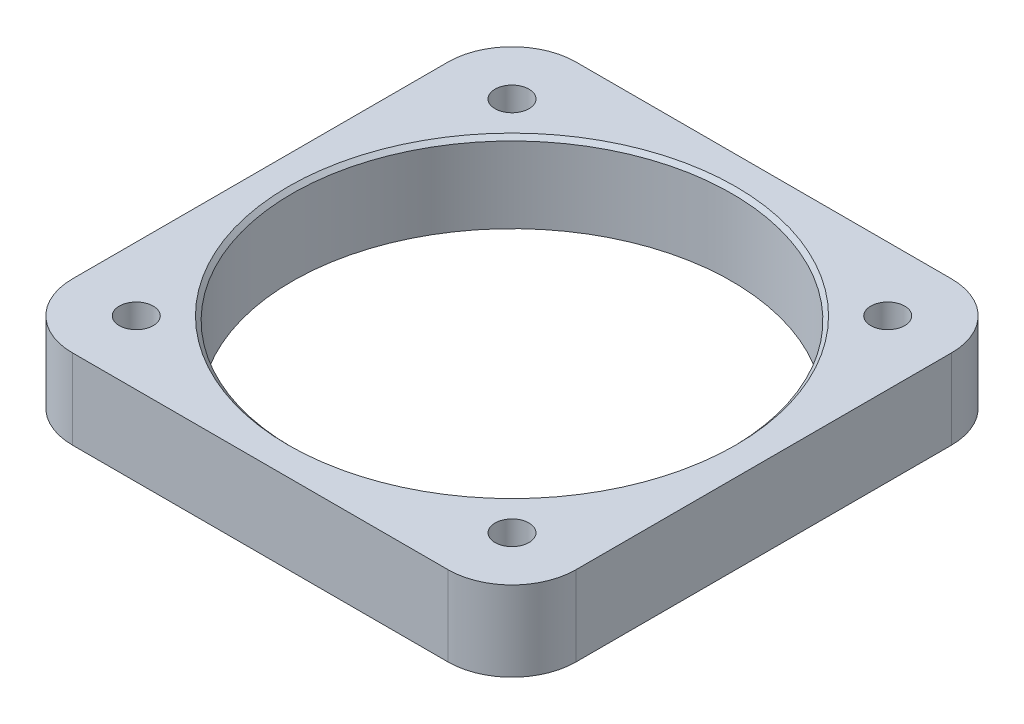
from build123d import *

# Parameters (mm, degrees)
SKETCH1_R              = 55
BOSS_EXTRUDE1_DEPTH    = 20
SKETCH2_R              = 4
CUT_EXTRUDE1_DEPTH     = 3
M10_TAPPED_HOLE1_D     = 8.5
M10_TAPPED_HOLE1_DEPTH = 15.23
M10_TAPPED_HOLE1_TIP   = 2.553657631
CHAMFER1_SIZE          = 1


with BuildPart() as part:
    # Sketch1 → Boss-Extrude1 (new body)
    with BuildSketch(Plane(origin=(0, 0, 0), x_dir=(1, 0, 0), z_dir=(0, 1, 0))):
        with BuildLine():
            Line((-47, 63), (47, 63))
            ThreePointArc((47, 63), (58.313708499, 58.313708499), (63, 47))
            Line((63, 47), (63, -47))
            ThreePointArc((63, -47), (58.313708499, -58.313708499), (47, -63))
            Line((47, -63), (-47, -63))
            ThreePointArc((-47, -63), (-58.313708499, -58.313708499), (-63, -47))
            Line((-63, -47), (-63, 47))
            ThreePointArc((-63, 47), (-58.313708499, 58.313708499), (-47, 63))
        make_face()
        with Locations(Location((0, 0, 0), (0, 0, 270))):
            Circle(SKETCH1_R, mode=Mode.SUBTRACT)
    extrude(amount=BOSS_EXTRUDE1_DEPTH)

    # Sketch2 → Cut-Extrude1 (cut)
    with BuildSketch(Plane(origin=(0, 20, 0), x_dir=(1, 0, 0), z_dir=(0, 1, 0))):
        with Locations(Location((-47, 47, 0), (0, 0, 270))):
            Circle(SKETCH2_R)
        with Locations(Location((47, 47, 0), (0, 0, 270))):
            Circle(SKETCH2_R)
        with Locations(Location((47, -47, 0), (0, 0, 270))):
            Circle(SKETCH2_R)
        with Locations(Location((-47, -47, 0), (0, 0, 270))):
            Circle(SKETCH2_R)
    extrude(amount=-CUT_EXTRUDE1_DEPTH, mode=Mode.SUBTRACT)

    # M10 Tapped Hole1
    with Locations(Plane(origin=(0, 20, 0), x_dir=(1, 0, 0), z_dir=(0, 1, 0))):
        with Locations((-47, 47), (47, 47), (47, -47), (-47, -47)):
            Hole(M10_TAPPED_HOLE1_D / 2, depth=M10_TAPPED_HOLE1_DEPTH)
            with Locations((0, 0, -(M10_TAPPED_HOLE1_DEPTH + M10_TAPPED_HOLE1_TIP / 2))):  # 118° drill point
                Cone(0, M10_TAPPED_HOLE1_D / 2, M10_TAPPED_HOLE1_TIP, mode=Mode.SUBTRACT)

    # Chamfer1
    chamfer1_edges = [part.edges().sort_by_distance(p)[0] for p in [
        (0, 20, -55),
    ]]
    chamfer(chamfer1_edges, length=CHAMFER1_SIZE)


solid = part.part
